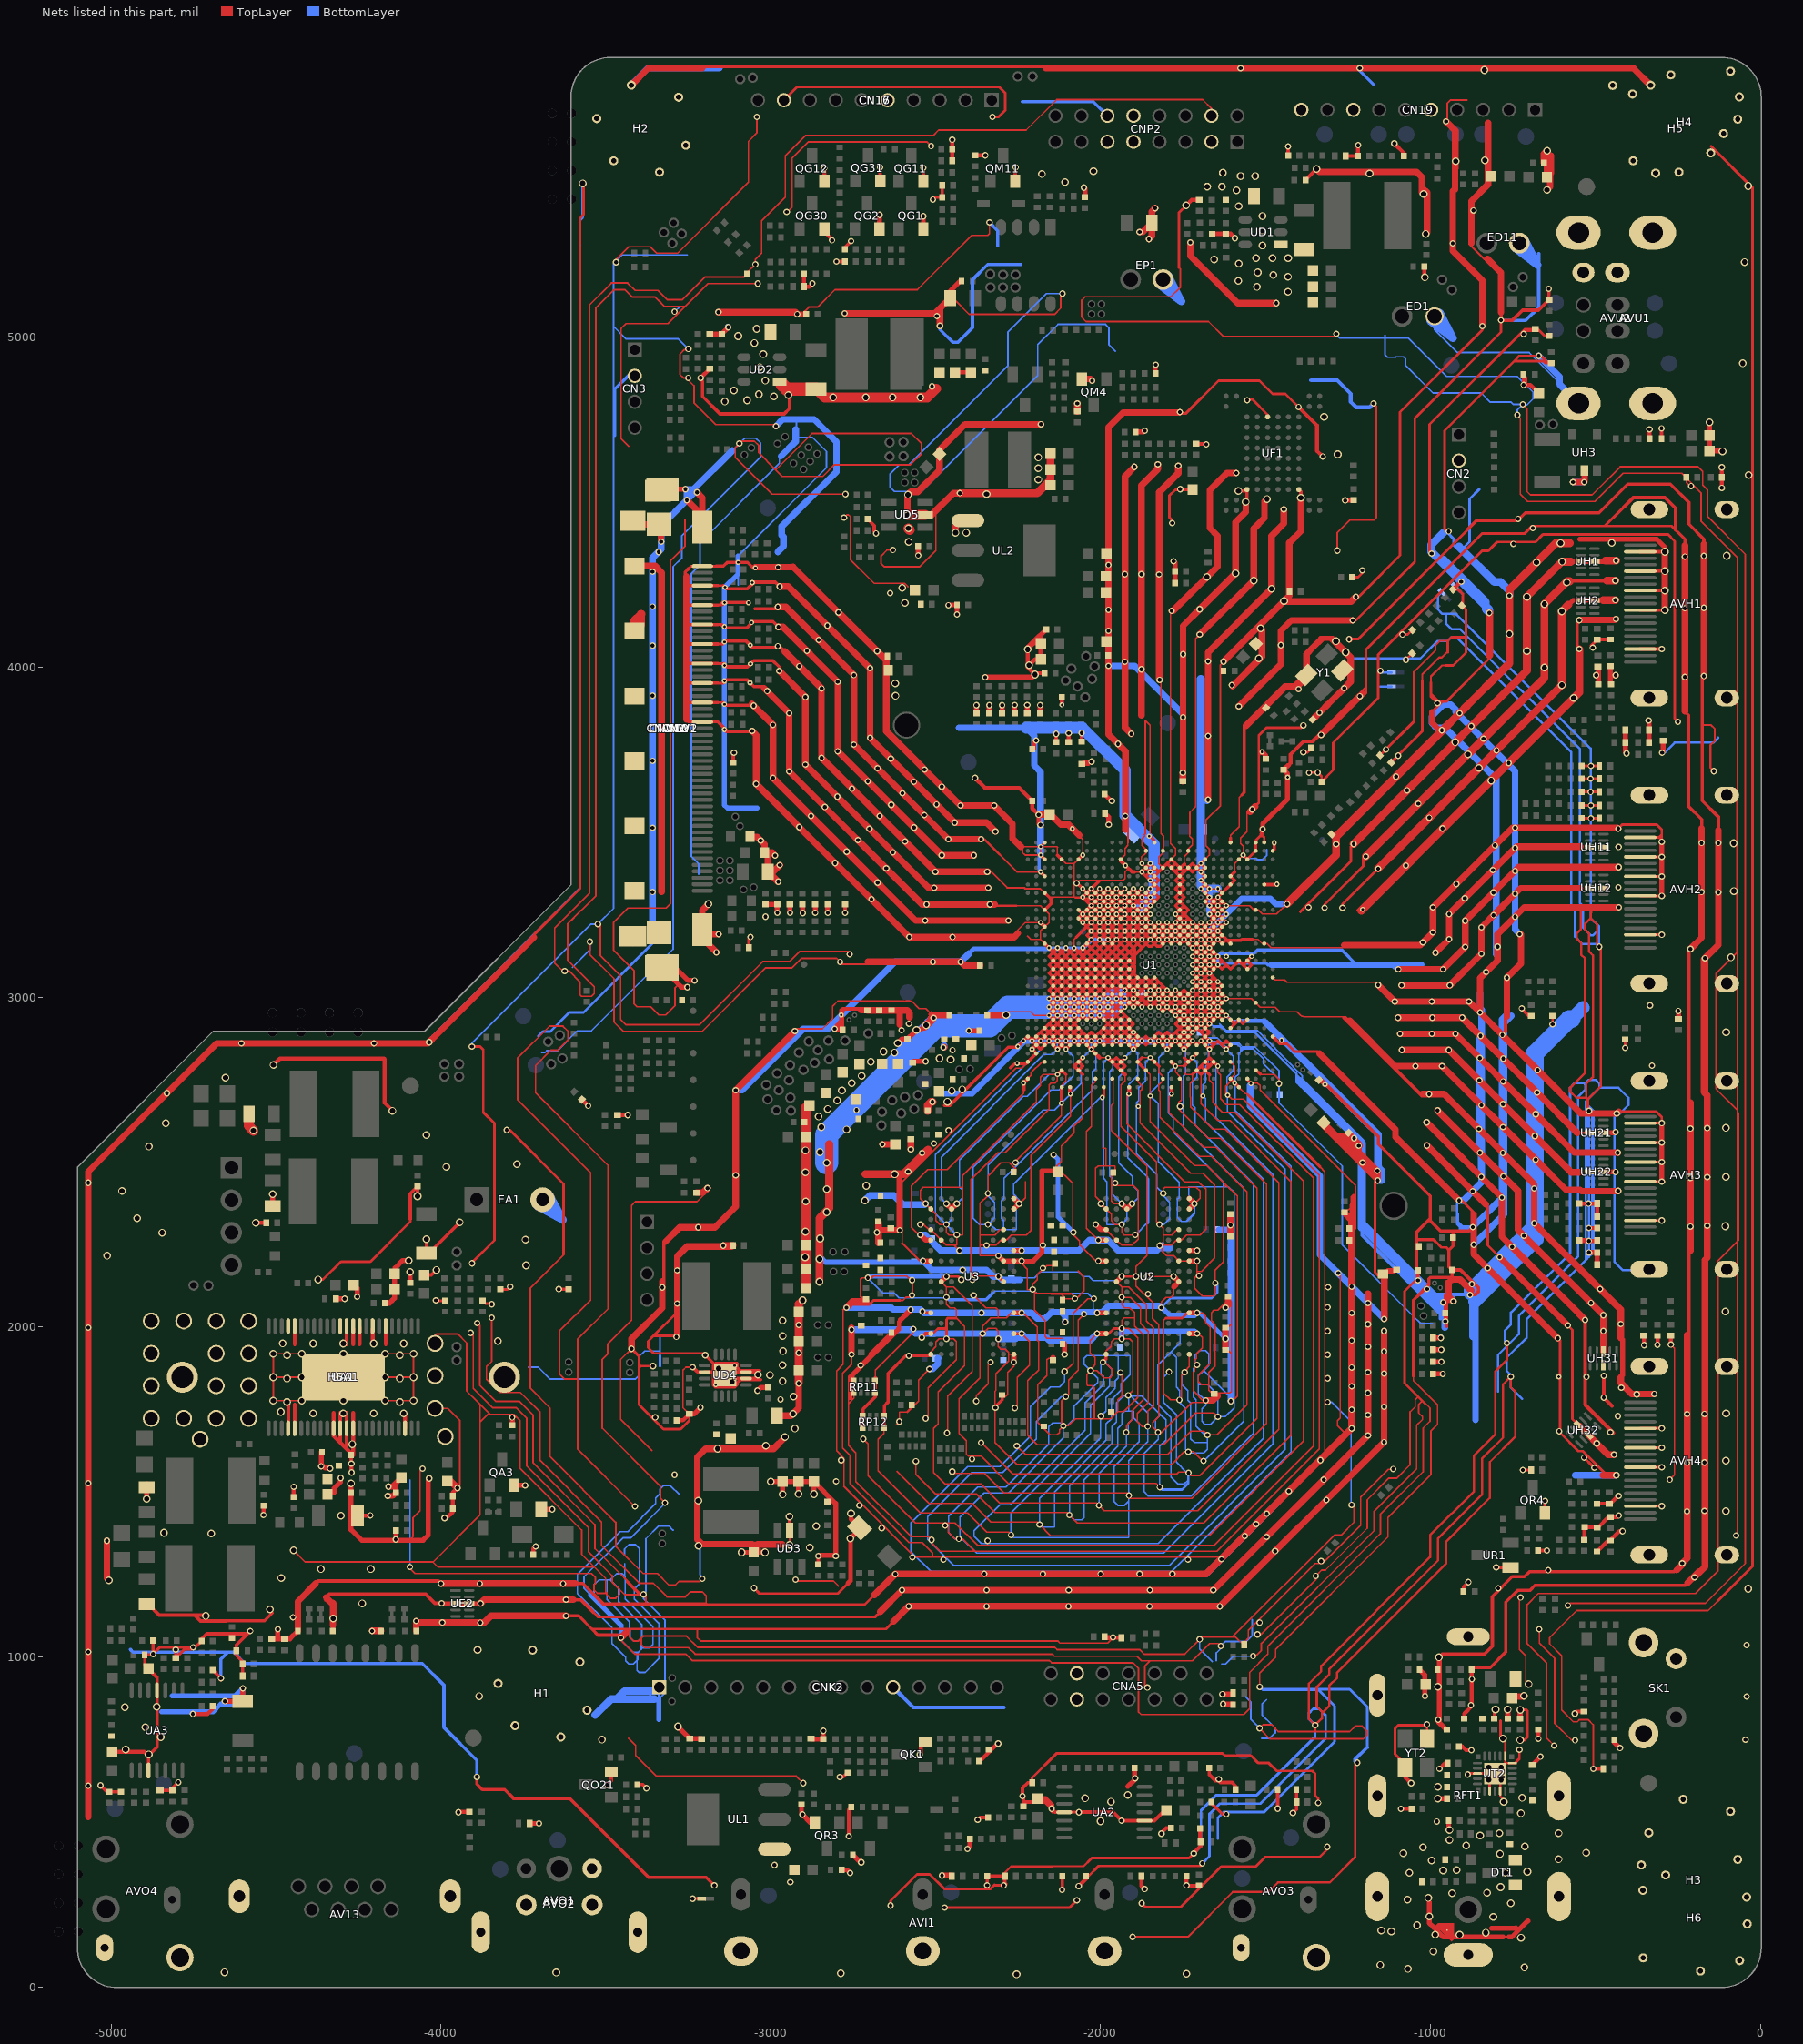
[diagram p0: the nets of this part, all layers, seen from the top]
# Altium PCB MISC86290.PcbDoc (part 14 of 31)
Units mil, origin at the board's own origin, x right, y up, seen from the top; angles counter-clockwise.
Board outline 5104.71 x 5851.49 mil, 2 copper layers (TopLayer, BottomLayer), stack 61.855 mil thick; 1026 components, 667 nets, 4280 pads, 2294 vias.

## Via types
v1: diameter 19.68, hole 11.81, TopLayer to BottomLayer, tented both sides, 1189 vias
v2: diameter 19.68/19.68 (per signal layer), hole 11.81, TopLayer to BottomLayer, tented both sides, 366 vias
v3: diameter 15.75, hole 7.87, TopLayer to BottomLayer, tented both sides, 348 vias
v4: diameter 23.62, hole 15.75, TopLayer to BottomLayer, tented both sides, 309 vias
v5: diameter 15.75/15.75 (per signal layer), hole 7.87, TopLayer to BottomLayer, tented both sides, 59 vias
v6: diameter 24/24 (per signal layer), hole 16, TopLayer to BottomLayer, tented both sides, 23 vias

## Nets (pads, with @x,y where several pads share a name; then routed paths per layer and width w, separated by ;. In a path a pad name is that pad's centre, name@x,y a point inside that pad or via, vN(x,y) a via of type N, cw(c..) or ccw(c..) an arc to the next point about the centre after c; other vN are vias at no path point) (continued)
GND: (continued)
  TopLayer w3.94: -2782.07,2050.79 -2774.2,2058.66 v2@-2772.23,2058.66 ; -2780.83,2050.79 -2780.83,1886.42 -2800.51,1866.73 -2800.51,1624.61 -2777.87,1601.97 -2777.87,1517.32 -2563.31,1302.76 -2509.17,1302.76 ; -2779.12,1517.32 v2@-2726.96,1465.16 ; -2759.72,1786.37 -2765.08,1781.02 -2765.08,1767.32 ; v2@-2755.24,1991.42 v2(-2755.24,1916.93) -2755.24,1886.42 -2782.8,1858.86 -2782.8,1633.46 -2760.16,1610.83 -2760.16,1525.2 -2581.02,1346.06 -2540.67,1346.06 -2509.17,1314.57 -2509.17,1302.76 ; v2(-2719.8,1661.02) -2705.04,1646.26 -2705.04,1548.82 -2562.32,1406.1 -2461.93,1406.1 ; C102.1@-2713.9,2078.35 -2727.68,2092.13 -2727.68,2145.28 -2723.74,2149.21 -2719.72,2149.21 ; C102.1@-2710.89,2078.35 -2715.15,2078.35 -2728.93,2092.12 -2728.93,2145.27 -2724.99,2149.21 -2720.97,2149.21 ; v2@-2707.27,2149.21 -2720.97,2149.21 ; v2(-2706.02,2149.21) -2719.72,2149.21 ; RP11.2@-2683.39,1800.79 -2683.39,1847.03 -2683.39,1868.7 -2568.23,1983.86 v2(-2568.23,1993.7) ; RP12.2@-2655.83,1694.49 -2656.81,1693.5 -2656.81,1677.76 -2675.51,1659.06 -2675.51,1564.57 -2546.57,1435.63 -2403.86,1435.63 -2345.79,1377.56 -2279.84,1377.56 v2(-2271.97,1369.69) ; -2618.43,1562.6 -2520.98,1465.16 -2390.08,1465.16 -2332.99,1408.07 -2192.24,1408.07 v2(-2185.35,1401.18) -2151.89,1367.72 -1671.57,1367.72 -1385.16,1654.13 -1385.16,2442.52 -1593.82,2651.18 -1631.22,2651.18 -1660.75,2680.71 -1660.75,2729.7 ; v2@-2610.55,1712.2 v2(-2610.55,1713.19) -2610.55,1742.72 -2585.63,1742.72 ; -2601.69,2254.53 -2601.69,2440.55 -2257.2,2785.04 -2239.49,2785.04 U1.D30@-2219.8,2804.72 ; -2589.97,2155.03 -2690.15,2155.03 -2695.97,2149.21 -2720.97,2149.21 ; v2(-2576.1,2052.76) -2576.1,2044.88 -2607.6,2013.39 -2607.6,1991.73 -2747.36,1851.97 -2747.36,1785.04 -2765.08,1767.32 ; v2@-2572.46,2095.77 -2572.46,2097.8 -2569.72,2100.53 -2569.72,2136.03 -2588.72,2155.03 -2688.91,2155.03 -2694.72,2149.21 -2719.72,2149.21 ; C103.1@-2564.96,1763.39 -2552.48,1775.87 -2552.48,1839.17 v2(-2519.02,1872.64) ; v2(-2560.35,1593.11) -2560.35,1553.74 -2501.3,1494.69 -2377.28,1494.69 -2320.2,1437.6 -2102.68,1437.6 v2(-2094.8,1429.72) -2071.18,1406.1 -1688.31,1406.1 -1422.56,1671.85 -1422.56,2440.55 -1607.6,2625.59 -1645,2625.59 -1696.18,2676.77 -1696.18,2765.35 ; v2@-2547.56,2200.39 v2(-2538.7,2200.39) ; v2(-2546.57,2279.13) -2551.5,2279.13 -2574.13,2301.77 -2574.13,2427.76 -2524.92,2476.97 -2465.87,2476.97 -2233.58,2709.25 -2233.58,2719.09 ; v2(-2530.83,1723.03) -2522.95,1730.91 -2522.95,1815.55 -2437.32,1901.18 -2437.32,1955.31 -2446.18,1964.17 v2(-2467.83,1964.17) -2489.49,1964.17 -2499.33,1954.33 -2499.33,1940.55 -2515.08,1924.8 U3.T1@-2515.08,1916.93 ; U3.P1@-2515.08,1979.92 U3.P1@-2509.17,1979.92 ; U3.D1@-2515.08,2294.88 -2467.83,2247.64 -2444.21,2247.64 ; U3.J2@-2483.58,2137.4 -2467.83,2121.65 ; -2473.74,1995.67 -2467.83,2001.57 ; v2(-2465.87,1678.74) -2463.9,1678.74 -2463.9,1789.96 -2389.09,1864.76 -2389.09,2064.57 -2446.18,2121.65 -2467.83,2121.65 ; v2(-2450.12,1561.61) -2442.24,1555.71 -2352.68,1555.71 -2293.62,1496.65 -1918,1496.65 v2(-1914.69,1488.78) -1915.67,1487.8 -1915.67,1480.91 -1723.74,1480.91 -1497.36,1707.28 -1497.36,2432.68 -1637.13,2572.44 -1674.53,2572.44 -1763.11,2661.02 -1763.11,2680.71 -1755.24,2688.58 -1755.24,2747.64 U1.B12@-1760.16,2752.56 -1760.16,2760.43 -1772.95,2773.23 v5(-1772.95,2790.94) -1747.36,2790.94 -1747.2,2790.78 -1747.2,2771.4 -1740.8,2765 -1721.77,2765 ; v2(-2428.46,2231.89) -2444.21,2247.64 ; v2(-2385.16,2096.06) -2347.76,2058.66 -2318.23,2058.66 -2310.35,2050.79 -2310.35,2027.17 ; v2(-2377.28,1775.2) -2377.28,1791.93 -2341.85,1827.36 -2341.85,1885.43 v2(-2333.98,1893.31) ; v2(-2362.52,1649.21) -2361.54,1649.21 -2267.05,1554.72 -1769.02,1554.72 -1763.11,1560.63 -1736.54,1560.63 v2@-1734.07,1558.17 ; v2(-2319.21,1755.51) v2@-2320.2,1757.54 ; v2(-2310.35,2153.15) -2314.29,2155.12 -2384.17,2155.12 -2393.03,2163.98 -2393.03,2447.44 -2312.32,2528.15 -2289.69,2528.15 -2156.81,2661.02 -2156.81,2733.86 -2150.91,2739.76 -2139.09,2739.76 -2131.22,2747.64 v5(-2131.22,2765.35) -2174.53,2765.35 -2182.4,2757.48 -2182.4,2732.87 -2195.2,2720.08 -2195.2,2682.68 -2418.62,2459.25 -2418.62,2422.83 ; v2(-2310.35,2216.14) -2365.47,2216.14 -2365.47,2247.64 ; C50.2@-2298.94,1787.48 -2290.2,1787.48 -2281.81,1795.87 -2281.81,1862.8 -2263.11,1881.5 v2(-2263.11,1893.31) ; U3.D8@-2294.61,2294.88 -2305.43,2294.88 -2321.18,2279.13 -2365.47,2279.13 ; U3.T9@-2263.11,1916.93 -2278.86,1916.93 ; U3.M9@-2263.11,2042.91 -2270.98,2042.91 -2286.73,2027.17 -2310.35,2027.17 ; v2(-2260.16,1754.53) -2260.16,1757.43 -2253.27,1763.34 -2253.27,1847.05 -2215.87,1884.45 -2215.87,1956.3 v2(-2239.49,1979.92) ; v2(-2258.19,2498.62) -2258.19,2502.56 -2119.41,2641.34 v5(-2119.41,2678.74) v5@-2118.43,2679.72 ; C76.1@-2257.2,2470.39 -2257.2,2477.95 -2276.89,2497.64 -2302.48,2497.64 -2341.85,2458.27 v2(-2341.85,2405.12) -2341.85,2399.21 -2365.47,2375.59 -2365.47,2279.13 ; -2255.71,3276.78 -2255.32,3277.17 -2182.4,3277.17 U1.AB28@-2169.61,3264.37 ; -2255.32,3381.43 -2253.42,3379.53 v3(-2182.4,3379.53) ; v2(-2254.25,1639.37) -2228.66,1613.78 -1796.57,1613.78 -1726.69,1683.66 -1687.32,1683.66 v2(-1676.5,1672.83) -1647.95,1672.83 -1556.42,1764.37 -1556.42,2409.06 -1664.69,2517.32 -1702.09,2517.32 -1820.2,2635.43 -1820.2,2714.17 -1824,2717.98 -1824,2733.01 -1811.34,2745.67 ; v2(-2247.36,2373.62) -2228.66,2392.32 -2228.66,2441.85 ; v2(-2239.49,2042.91) -2234.57,2042.91 -2192.24,2000.59 -2192.24,1960.24 -2188.31,1956.3 -2188.31,1869.69 -2220.79,1837.2 -2220.79,1671.85 -2192.24,1643.31 -1809.37,1643.31 -1712.91,1739.76 -1656.81,1739.76 v2(-1645,1727.95) ; v2(-2239.49,2200.39) -2239.49,2192.52 -2222.26,2175.3 -2222.26,2113.78 v2@-2207.01,2113.78 ; -2222,3185.5 -2211.3,3174.8 -2182.4,3174.8 ; U1.B30@-2220.79,2752.56 -2210.94,2762.4 -2210.94,2770.28 -2177.48,2803.74 U1.D28@-2169.61,2803.74 ; U1.V28@-2169.61,3162.01 -2182.4,3174.8 ; U1.Y28@-2169.61,3213.19 -2182.4,3200.39 -2182.4,3174.8 ; -2156.81,3302.76 -2143.03,3302.76 ; -2152,2101.97 -2149.42,2099.39 -2092.47,2099.39 -2089.88,2101.97 ; -2150.91,3294.88 -2143.03,3302.76 ; -2145.32,2170.55 C73.1@-2145.32,2192.52 ; C73.1@-2145.32,2186.61 -2163.7,2186.61 -2192.24,2158.07 -2192.24,2143.31 -2206.02,2129.53 v2(-2206.02,2113.78) ; C42.2@-2145,1905.43 -2145.41,1905.02 -2158.19,1905.02 -2162.72,1900.5 -2162.72,1852.95 -2190.28,1825.39 -2190.28,1709.92 -2172.56,1692.2 -2153.19,1672.83 -2133.19,1672.83 -2125.32,1680.71 -2125.32,1688.58 v2(-2113.5,1700.39) ; -2119.41,2100 -2109.57,2090.16 R100.1@-2109.57,2082.6 ; v2@-2118.43,1705.31 v2(-2113.5,1700.39) ; -2118.43,1776.18 v2(-2105.63,1788.98) -2097.76,1796.85 -2097.76,1839.17 -2068.23,1868.7 -2068.23,2021.26 v2(-2050.51,2038.98) ; U1.A26@-2118.43,2726.97 -2118.43,2732.87 -2105.63,2745.67 -2105.63,2765.35 ; -2114,1966.14 -2162.72,1966.14 -2168.62,1972.05 -2168.62,2019.29 -2200.12,2050.79 v2@-2200.12,2107.87 ; v2(-2109.57,1864.76) -2083.98,1890.35 -2083.98,2041.93 -2039.69,2086.22 v2(-2020.98,2086.22) ; v2(-2109.57,1916.93) v2@-2109.25,1917.24 ; R100.1@-2109.25,2082.28 R100.1@-2109.57,2082.6 ; v5@-2092.83,2706.3 v5(-2091.85,2706.3) -2091.85,2639.37 -2210.94,2520.28 -2210.94,2292.91 -2224.72,2279.13 -2270.98,2279.13 -2286.73,2263.39 -2302.48,2263.39 -2318.23,2247.64 v2(-2345.79,2247.64) -2365.47,2247.64 ; -2070.2,2170.55 -2050.51,2150.87 -2050.51,2109.84 v2@-2074.13,2086.22 ; U1.AH24@-2067.24,3417.91 -2080.04,3405.12 -2080.04,3304.72 ; -2054.45,2765.35 -2054.45,2745.67 -2056.42,2743.7 -2056.42,2632.48 -2080,2608.9 -2080,2588.5 -2119.41,2549.09 -2119.41,2501.57 -2135.16,2485.83 -2084.96,2435.63 -2084.96,2281.1 -2064.29,2260.43 -2064.29,2249.61 -2015.08,2200.39 v2(-2007.2,2200.39) ; v3(-2054.45,3302.76) -2080.04,3302.76 ; -2019.02,1814.57 -2026.89,1822.44 -2038.7,1822.44 -2042.64,1826.38 -2042.64,1855.91 v2(-2030.83,1867.72) ; U1.B22@-2016.06,2752.56 -2016.06,2744.68 -2028.86,2731.89 -2028.86,2607.87 -2043.62,2593.11 -2043.62,2299.8 v2(-2007.2,2263.39) ; U1.AC22@-2016.06,3289.96 -2017.05,3288.98 -2019.02,3288.98 -2030.83,3300.79 -2076.1,3300.79 -2080.04,3304.72 ; v2(-2011.14,1979.92) -2031.81,1959.25 -2031.81,1921.85 -2017.05,1907.09 -2017.05,1885.43 v2(-2030.83,1867.72) ; -2003.27,2816.54 v5(-1977.68,2816.54) ; v5(-1995.39,2695.47) -1995.39,2690.55 -1993.43,2688.58 -1993.43,2541.93 -1983.58,2541.93 -1983.58,2488.78 ; v2(-1993.43,1893.31) -1991.46,1891.34 -1985.55,1891.34 -1965.87,1871.65 -1965.87,1851.97 -1971.77,1846.06 -1989.49,1846.06 -2011.14,1867.72 v2(-2030.83,1867.72) ; U2.T1@-1983.58,1916.93 -1983.58,1926.77 -1967.83,1942.52 -1967.83,1954.33 -1957.99,1964.17 v2(-1936.34,1964.17) v2@-1932.4,1964.17 ; U2.P1@-1983.58,1979.92 -1975.71,1979.92 ; U2.D1@-1983.58,2294.88 U2.E2@-1952.09,2263.39 -1936.34,2247.64 -1904.84,2247.64 -1886.14,2266.34 -1886.14,2413.98 -1900.91,2428.74 -1967.83,2428.74 ; U1.B20@-1964.88,2752.56 -1962.14,2749.81 -1962.14,2677.55 -1967.83,2671.85 -1967.83,2595.08 -1860.55,2487.8 -1860.55,2216.14 -1893.03,2183.66 v2(-1893.03,2153.15) -1893.03,2124.61 -1843.82,2075.39 -1843.82,2026.18 -1824.13,2006.5 -1824.13,1727.95 -1841.85,1710.24 -1841.85,1696.46 v2(-1826.1,1680.71) ; U2.J2@-1952.09,2137.4 -1936.34,2121.65 ; -1952.09,2790.94 U1.C19@-1939.29,2778.15 ; v2(-1940.28,1861.81) -1940.28,1859.84 -1936.34,1855.91 -1936.34,1790.94 -1948.15,1779.13 -1948.15,1743.7 ; U1.D19@-1940.28,2802.76 v5(-1926.5,2816.54) ; U1.AH19@-1939.29,3417.91 -1926.5,3430.71 -1926.5,3451.26 -1917.22,3460.53 -1917.22,3468.11 ; v2(-1936.34,2373.62) -1959.96,2373.62 -1967.83,2381.5 -1967.83,2428.74 ; -1926.5,2765.35 -1926.5,2745.67 -1938.31,2733.86 -1938.31,2607.87 -1831.02,2500.59 -1831.02,2319.49 v2(-1822.17,2310.63) -1810.35,2298.82 -1810.35,2279.13 ; v2(-1916.65,1792.91) -1902.87,1806.69 -1902.87,1954.33 -1912.72,1964.17 v2@-1932.4,1964.17 ; v5(-1914.69,2706.3) -1920.59,2700.39 -1920.59,2615.75 -1745.39,2440.55 -1704.06,2440.55 -1681.42,2417.91 -1681.42,2295.87 -1698.15,2279.13 -1739.49,2279.13 -1755.24,2263.39 U2.E8@-1763.11,2263.39 -1770,2263.39 -1785.75,2247.64 v2@-1814.29,2247.64 ; v2(-1895,2279.13) -1928.46,2279.13 -1936.34,2287.01 v2(-1936.34,2310.63) -1956.02,2310.63 -1967.83,2322.44 -1967.83,2342.13 v2(-1999.33,2373.62) -1999.33,2379.53 -2016.06,2396.26 -2016.06,2480.91 -2008.19,2488.78 -1983.58,2488.78 ; U1.B17@-1888.11,2752.56 -1888.11,2744.18 -1875,2731.07 -1875,2720.39 -1880.24,2715.16 -1880.24,2618.7 -1727.68,2466.14 -1690.28,2466.14 -1653.86,2429.72 -1653.86,2209.25 -1694.21,2168.9 -1707.99,2168.9 ; -1875.32,2816.54 v5(-1849.72,2816.54) ; -1867.22,3492.35 -1867.22,3488.01 -1875.32,3479.92 -1875.32,3460.24 U1.AJ16@-1862.52,3447.44 ; U1.C16@-1862.52,2778.15 -1849.72,2765.35 v5(-1849.72,2700.39) -1849.72,2623.62 -1715.87,2489.76 -1678.46,2489.76 -1619.41,2430.71 ; U1.AG16@-1862.52,3392.32 -1875.94,3405.75 -1875.94,3423.83 -1862.52,3437.25 U1.AJ16@-1862.52,3443.5 ; v2(-1859.57,2153.15) v2(-1778.86,2153.15) ; -1824.5,2788.61 -1824.5,2772.87 -1811.34,2759.71 U1.B14@-1811.34,2752.56 ; v2(-1821.18,1514.37) -1832.99,1526.18 -2280.83,1526.18 -2362.52,1607.87 -2400.91,1607.87 -2406.81,1613.78 -2406.81,1655.12 -2429.45,1677.76 -2429.45,1782.09 -2365.47,1846.06 -2365.47,1972.05 v2(-2357.6,1979.92) ; -1817.22,3506.05 -1817.22,3496.63 -1808.39,3487.8 -1808.39,3453.35 -1811.34,3450.39 -1811.34,3436.61 -1824.13,3423.82 -1824.13,3405.12 U1.AG14@-1811.34,3392.32 ; v2(-1816.26,2058.66) -1816.26,2076.38 -1802.48,2090.16 -1786.73,2090.16 -1778.86,2098.03 -1778.86,2121.65 ; v2(-1810.35,2405.12) -1810.35,2418.9 -1805.43,2423.82 -1710.94,2423.82 -1699.13,2412.01 -1699.13,2390.35 v2(-1715.87,2373.62) ; -1802.48,2027.17 -1808.39,2021.26 -1808.39,1798.82 -1788.7,1779.13 v2(-1761.14,1779.13) -1755.24,1785.04 -1755.24,1852.95 v2(-1745.39,1862.8) -1743.43,1867.72 -1731.61,1879.53 U2.T9@-1731.61,1916.93 ; v5(-1785.75,2706.3) -1786.73,2704.33 -1792.64,2698.43 -1792.64,2649.21 -1688.31,2544.88 -1650.91,2544.88 -1526.89,2420.87 -1526.89,1723.03 -1700.12,1549.8 -1726.69,1549.8 -1734.07,1557.19 v2@-1734.07,1558.17 ; U1.AH13@-1785.75,3417.91 -1772.95,3430.71 -1772.95,3450.39 -1784.76,3462.2 ; U2.D8@-1763.11,2294.88 -1769.02,2294.88 -1784.76,2279.13 -1810.35,2279.13 ; -1747.36,2816.54 v5(-1747.36,2842.13) ; -1746.73,3404.49 -1746.73,3425.43 -1746.38,3425.79 -1734.57,3437.6 -1734.57,3449.41 -1721.77,3462.2 -1721.77,3480.08 -1729.72,3488.03 -1729.72,3494.43 ; -1746.38,3404.13 U1.AG11@-1734.57,3392.32 ; v2(-1733.58,1557.68) v2@-1734.07,1558.17 ; U2.G9@-1731.61,2200.39 U2.G8@-1763.11,2200.39 -1778.86,2216.14 -1800.51,2216.14 -1814.29,2229.92 v2@-1814.29,2247.64 ; -1721.77,2765.35 -1721.77,2765 ; v2(-1707.99,1979.92) -1704.06,1979.92 -1692.24,1968.11 -1692.24,1936.61 -1709.96,1918.9 -1709.96,1905.12 -1715.87,1899.21 -1715.87,1865.75 -1719.8,1861.81 -1719.8,1806.69 -1684.37,1771.26 v2@-1680.4,1771.26 ; v2(-1707.99,2042.91) -1692.24,2042.91 -1682.4,2033.07 -1682.4,2013.39 -1668.62,1999.61 -1668.62,1889.37 -1704.06,1853.94 -1704.06,1834.25 -1694.21,1824.41 -1672.56,1824.41 ; v2(-1707.99,2200.39) -1707.99,2168.9 ; v2(-1688.31,1594.09) -1692.24,1594.09 -1719.8,1621.65 v2(-1734.57,1621.65) -1746.38,1621.65 -1783.78,1584.25 -2254.25,1584.25 -2320.2,1650.2 v2@-2320.2,1757.54 ; -1680.43,3459.14 -1680.43,3537.01 -1637.22,3580.22 ; -1671,2762.98 -1671,2748.56 -1660.75,2738.3 -1660.75,2729.7 ; v5(-1670.59,2842.13) -1670.59,2816.54 v5(-1645,2790.94) ; v3(-1670.59,3328.35) v3(-1645,3328.35) ; -1660.71,2729.74 -1660.75,2729.7 ; C74.1@-1646.36,1790.53 -1646.13,1790.53 -1636.86,1799.8 ; v5@-1644.02,2789.96 v5(-1645,2790.94) ; R67.1@-1621.38,1936.93 -1603.66,1919.21 -1603.66,1912.03 ; C99.1@-1621.38,1991.42 -1603.66,2009.13 -1603.66,2015.03 ; v3(-1619.41,3277.17) -1548.17,3277.17 -1535.37,3264.37 U1.AB3@-1529.84,3264.37 -1522.12,3264.37 -1509.19,3251.43 -1467.5,3251.43 v1@-1435.84,3283.09 ; v3@-1619.34,2995.74 v3@-1619.25,2995.64 ; U1.AE6@-1608.58,3339.17 U1.AE6@-1606.61,3341.14 ; U1.B6@-1606.61,2752.56 -1606.68,2752.49 -1607.6,2751.57 -1607.6,2743.7 -1621.38,2729.92 -1621.38,2704.33 -1615.47,2698.43 v5(-1615.47,2702.36) -1613.59,2701.96 -1602.18,2690.55 -1568.23,2690.55 -1337.91,2460.24 -1337.91,1630.51 -1647.95,1320.47 -2381.22,1320.47 ; U1.AF6@-1606.61,3366.73 U1.AF6@-1604.65,3368.7 ; U1.AK6@-1606.61,3469.09 -1606.61,3490.75 -1580.04,3517.32 -1580.04,3605.72 -1572.03,3613.73 ; v2(-1605.63,1775.2) -1601.69,1775.2 -1585.94,1790.94 -1585.94,2397.24 -1619.41,2430.71 ; v3(-1568.23,3430.71) -1568.23,3458.23 -1576.1,3466.1 -1576.1,3481.89 -1556.42,3501.57 -1556.42,3562.51 v1@-1548.67,3570.26 ; v3(-1544.61,2737.8) -1544.32,2738.08 -1542.64,2739.76 -1524.92,2739.76 -1517.05,2731.89 -1517.05,2718.11 -1227.72,2428.78 ; U1.C3@-1529.84,2778.15 -1517.05,2765.35 -1474.81,2765.35 ; U1.L3@-1529.84,2982.87 -1516.65,2969.68 -1471.38,2969.68 -1457.99,2956.3 -1404.9,2956.3 -1393.31,2944.71 ccw(c-1384.36,2953.65) -1384.36,2941 -1257.69,2941 -1245,2928.31 ; U1.V2@-1504.25,3162.01 -1496.12,3162.01 -1483.94,3149.82 -1259.31,3149.82 -1251.27,3157.85 ; -1499,2765.35 -1498.37,2764.73 -1473.62,2764.73 -1459.22,2750.33 v2(-1459.22,2737.78) ; U1.G1@-1478.66,2880.51 U1.G1@-1475.71,2877.56 ; U1.P1@-1478.66,3059.65 -1470.62,3051.6 -1442.6,3051.6 -1435.88,3044.88 -1166.61,3044.88 v1@-1151.92,3030.19 ; -1351.01,3355.1 -1345,3361.11 ; -1334.55,2485.22 -1320.2,2470.87 -1320.2,1622.64 -1640.08,1302.76 -2509.17,1302.76 ; C13.2@-1260.94,2345.88 -1258.12,2345.88 -1235.75,2368.25 -1227.72,2376.28 ; -1230.69,2289 -1230.69,2295.08 -1227.72,2298.06 -1227.72,2376.28 ; -1227.72,2428.13 -1227.72,2376.28 ; -2765.08,1767.32 -2765.08,1641.34 -2741.85,1618.11 -2741.85,1531.5 -2574.13,1363.78 -2521.97,1363.78 v2(-2513.11,1354.92) -2513.11,1346.06 -2487.52,1320.47 -2381.22,1320.47 ; -2467.83,2121.65 v2(-2467.83,2090.16) -2467.83,2069 -2456.91,2058.07 -2443.43,2058.07 -2438.31,2052.95 -2438.31,2027.17 -2412.72,2001.57 -2412.72,1883.46 -2493.43,1802.76 -2493.43,1706.3 -2507.2,1692.52 -2507.2,1558.66 -2472.76,1524.21 -2363.5,1524.21 -2306.42,1467.13 -2013.11,1467.13 v2(-2005.24,1459.25) -1989.49,1443.5 -1706.02,1443.5 -1459.96,1689.57 -1459.96,2436.61 -1623.35,2600 -1660.75,2600 -1727.68,2666.93 -1727.68,2696.46 -1729.65,2698.43 -1729.65,2737.8 -1721.77,2745.67 -1721.77,2765 ; -2461.93,1406.1 -2461.93,1377.56 -2442.24,1357.87 v2(-2430.43,1357.87) -2418.62,1357.87 -2381.22,1320.47 ; -2461.93,1406.1 -2441.26,1406.1 -2373.35,1338.19 -1655.83,1338.19 -1355.63,1638.39 -1355.63,2452.36 -1578.07,2674.8 -1619.41,2674.8 -1637.13,2692.52 -1637.13,2763.68 -1645,2771.56 v5(-1645,2790.94) ; -2444.21,2247.64 -2436.34,2247.64 v2(-2436.34,2279.13) ; v2(-2436.34,2279.13) -2418.62,2279.13 -2418.62,2422.83 ; v2(-2436.34,2279.13) -2459.96,2279.13 -2467.83,2287.01 -2467.83,2306.69 -2471.77,2310.63 -2487.52,2310.63 -2499.33,2322.44 -2499.33,2342.13 U3.B1@-2515.08,2357.87 v2(-2530.83,2373.62) -2546.57,2389.37 -2546.57,2413.98 -2537.72,2422.83 -2418.62,2422.83 ; -2365.47,2247.64 -2365.47,2279.13 ; v2(-2357.6,1979.92) -2357.6,2002.56 -2332.99,2027.17 -2310.35,2027.17 ; v2(-2357.6,1979.92) -2341.85,1995.67 -2318.23,1995.67 -2310.35,1987.8 v2(-2310.35,1964.17) -2310.35,1940.55 -2302.48,1932.68 -2288.7,1932.68 -2278.86,1922.83 -2278.86,1916.93 ; v2@-2320.2,1757.54 -2320.2,1805.71 -2318.23,1807.68 -2318.23,1857.87 -2278.86,1897.24 -2278.86,1916.93 ; v2@-2207.01,2113.78 -2206.02,2112.8 v2(-2206.02,2113.78) ; v2@-2207.01,2113.78 v2(-2206.02,2113.78) ; v2(-2206.02,2113.78) v2@-2200.12,2107.87 ; v2@-2200.12,2107.87 -2194.21,2101.97 -2089.88,2101.97 ; -2143.03,3302.76 -2080.04,3302.76 ; v2(-2113.5,1700.39) -2098.74,1700.39 -2077.09,1722.05 -2019.02,1722.05 -1969.8,1722.05 -1948.15,1743.7 ; R100.1@-2109.57,2082.6 -2109.57,2086.22 v2(-2078.07,2086.22) v2@-2074.13,2086.22 ; -2089.88,2101.97 v2@-2074.13,2086.22 ; -2080.04,3302.76 -2080.04,3304.72 ; -1983.58,2488.78 -1955.87,2488.78 -1955.87,2467.95 -1955.71,2468.11 -1967.52,2456.3 -1967.83,2456.3 -1967.83,2428.74 ; -1948.15,1743.7 -1930.43,1743.7 -1887.13,1787.01 -1887.13,1967.13 -1915.67,1995.67 v2(-1936.34,1995.67) ; v2(-1936.34,1995.67) -1940.28,1995.67 -1936.34,1991.73 -1936.34,1968.11 v2@-1932.4,1964.17 ; v2(-1936.34,1995.67) -1936.34,2019.29 -1928.46,2027.17 -1896.97,2027.17 ; v2(-1936.34,2090.16) -1909.76,2090.16 -1879.25,2059.65 -1879.25,2010.43 -1855.63,1986.81 -1855.63,1771.26 -1889.09,1737.8 -1889.09,1713.19 -1874.33,1698.43 v2(-1857.6,1698.43) -1857.6,1744.34 -1839.88,1762.06 -1839.88,1996.65 -1861.54,2018.31 -1861.54,2067.52 -1915.67,2121.65 -1936.34,2121.65 ; v2(-1936.34,2090.16) -1936.34,2121.65 ; v2(-1936.34,2090.16) -1936.34,2067.52 -1927.48,2058.66 -1911.73,2058.66 -1896.97,2043.9 -1896.97,2027.17 ; -1896.97,2027.17 -1896.97,2002.56 -1871.38,1976.97 -1871.38,1779.13 -1904.84,1745.67 -1904.84,1718.11 -1922.56,1700.39 v2(-1922.56,1680.71) -1922.56,1672.83 -1822.17,1672.83 -1723.74,1771.26 v2@-1680.4,1771.26 ; v2@-1814.29,2247.64 -1810.35,2251.57 -1810.35,2279.13 ; -1707.99,2168.9 -1707.99,2157.09 -1715.87,2149.21 -1715.87,2117.72 -1692.24,2094.09 -1656.81,2094.09 -1652.87,2098.03 v2(-1652.87,2133.46) -1652.87,2172.83 -1628.27,2197.44 -1628.27,2421.85 -1619.41,2430.71 ; v2@-1680.4,1771.26 -1676.5,1771.26 C74.1@-1655.98,1791.77 ; -1672.56,1824.41 -1672.56,1808.35 C74.1@-1655.98,1791.77 ; -1672.56,1824.41 -1672.56,1861.81 -1652.87,1881.5 -1652.87,2007.48 -1664.69,2019.29 -1664.69,2042.91 -1656.81,2050.79 -1645,2050.79 -1617.44,2078.35 -1613.5,2085.91 -1603.66,2076.06 -1603.66,2015.03 ; C74.1@-1655.98,1791.77 -1654.84,1790.63 -1652.87,1794.57 -1652.87,1799.8 -1636.86,1799.8 ; -1636.86,1799.8 -1608.58,1799.8 -1603.66,1804.72 -1603.66,1912.03 ; -1603.66,1912.03 -1603.66,2015.03
  TopLayer w4: v3(-2080.52,3148.73) -2080.52,3175.48 -2042.81,3213.19
  TopLayer w4.33: -1555.43,3174.8 -1522.95,3174.8 -1510.16,3162.01 U1.V2@-1504.25,3162.01
  TopLayer w4.92: -2237,3461.11 -2237,3444 -2237,3438.74 -2229.1,3430.84 v3@-2182.54,3430.84 ; -2234.3,3456.3 -2133.3,3456.3 ; v3(-2182.4,3456.3) v3(-2182.4,3430.71) v3@-2181.91,3430.22 ; -2131.36,3430.84 -2131.36,3454.36 -2133.3,3456.3 ; -2130.79,3430.28 -2105.63,3405.12 -2080.04,3405.12 ; -2130.73,3453.73 -2133.3,3456.3 ; U1.AD7@-1632.2,3315.55 U1.AE6@-1608.58,3339.17 ; -1593.68,3379.66 -1593.68,3405.25 U1.AH5@-1581.02,3417.91 v3(-1568.23,3430.71)